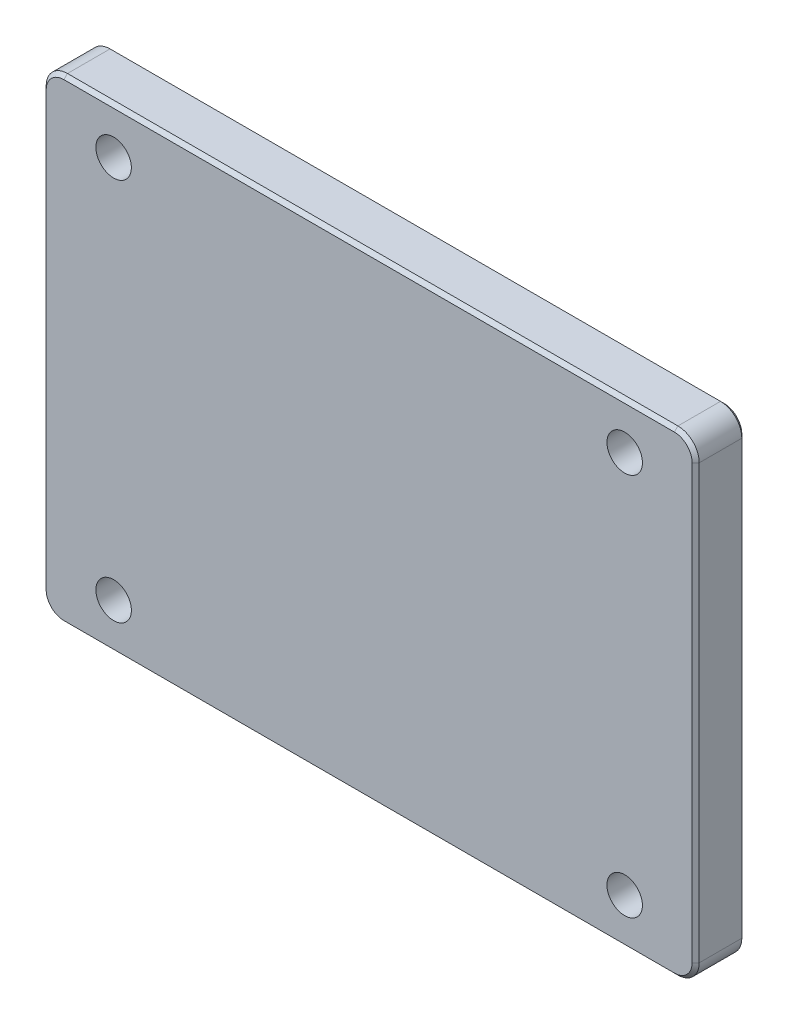
SolidWorks part; units mm, degrees
ref_plane "前视" through (0, 0, 0) normal (0, 0, 1) x (1, 0, 0)
ref_plane "上视" through (0, 0, 0) normal (0, 1, 0) x (1, 0, 0)
ref_plane "右视" through (0, 0, 0) normal (1, 0, 0) x (0, 0, -1)
sketch "草图1" plane through (0, 0, 0) normal (0, 0, 1) x (1, 0, 0)
  line L1 (-46, -33.5) -> (46, -33.5)
  line L2 (-46, -33.5) -> (-46, 33.5)
  line L3 (-46, 33.5) -> (46, 33.5)
  line L4 (46, -33.5) -> (46, 33.5)
  line L5 (-46, -33.5) -> (46, 33.5) construction
  line L6 (-46, 33.5) -> (46, -33.5) construction
  point P0 (0, 0)
  dimension "D1" = 92
  dimension "D2" = 67
extrude "凸台-拉伸1" add sketch "草图1" along normal blind 7
fillet "圆角1" radius 3 4 edges at (46, -33.5, 3.5) (-46, -33.5, 3.5) (46, 33.5, 3.5) (-46, 33.5, 3.5)
sketch "草图2" plane through (0, 0, 7) normal (0, 0, 1) x (1, 0, 0)
  line L0 (0, 0) -> (0, 29.7093) construction
  line L1 (0, 0) -> (-31.3333, 0) construction
  circle A0 centre (-36, 27) radius 2.5
  dimension "D1" = 5
  dimension "D3" = 54
  dimension "D2" = 36
extrude "切除-拉伸1" cut sketch "草图2" against normal blind 10
pattern_linear "阵列(线性)1" count 2 spacing 72 along (1, 0, 0) count 2 spacing 54 along (0, -1, 0) of "切除-拉伸1"
chamfer "倒角1" distance 0.5 angle 45 16 edges at (46, 0, 0) (45.1213, 32.6213, 0) (45.1213, -32.6213, 0) (0, 33.5, 0) (0, -33.5, 0) (-45.1213, 32.6213, 0) (-45.1213, -32.6213, 0) (-46, 0, 0) (46, 0, 7) (45.1213, 32.6213, 7) (45.1213, -32.6213, 7) (0, 33.5, 7) (0, -33.5, 7) (-45.1213, 32.6213, 7) (-45.1213, -32.6213, 7) (-46, 0, 7)
